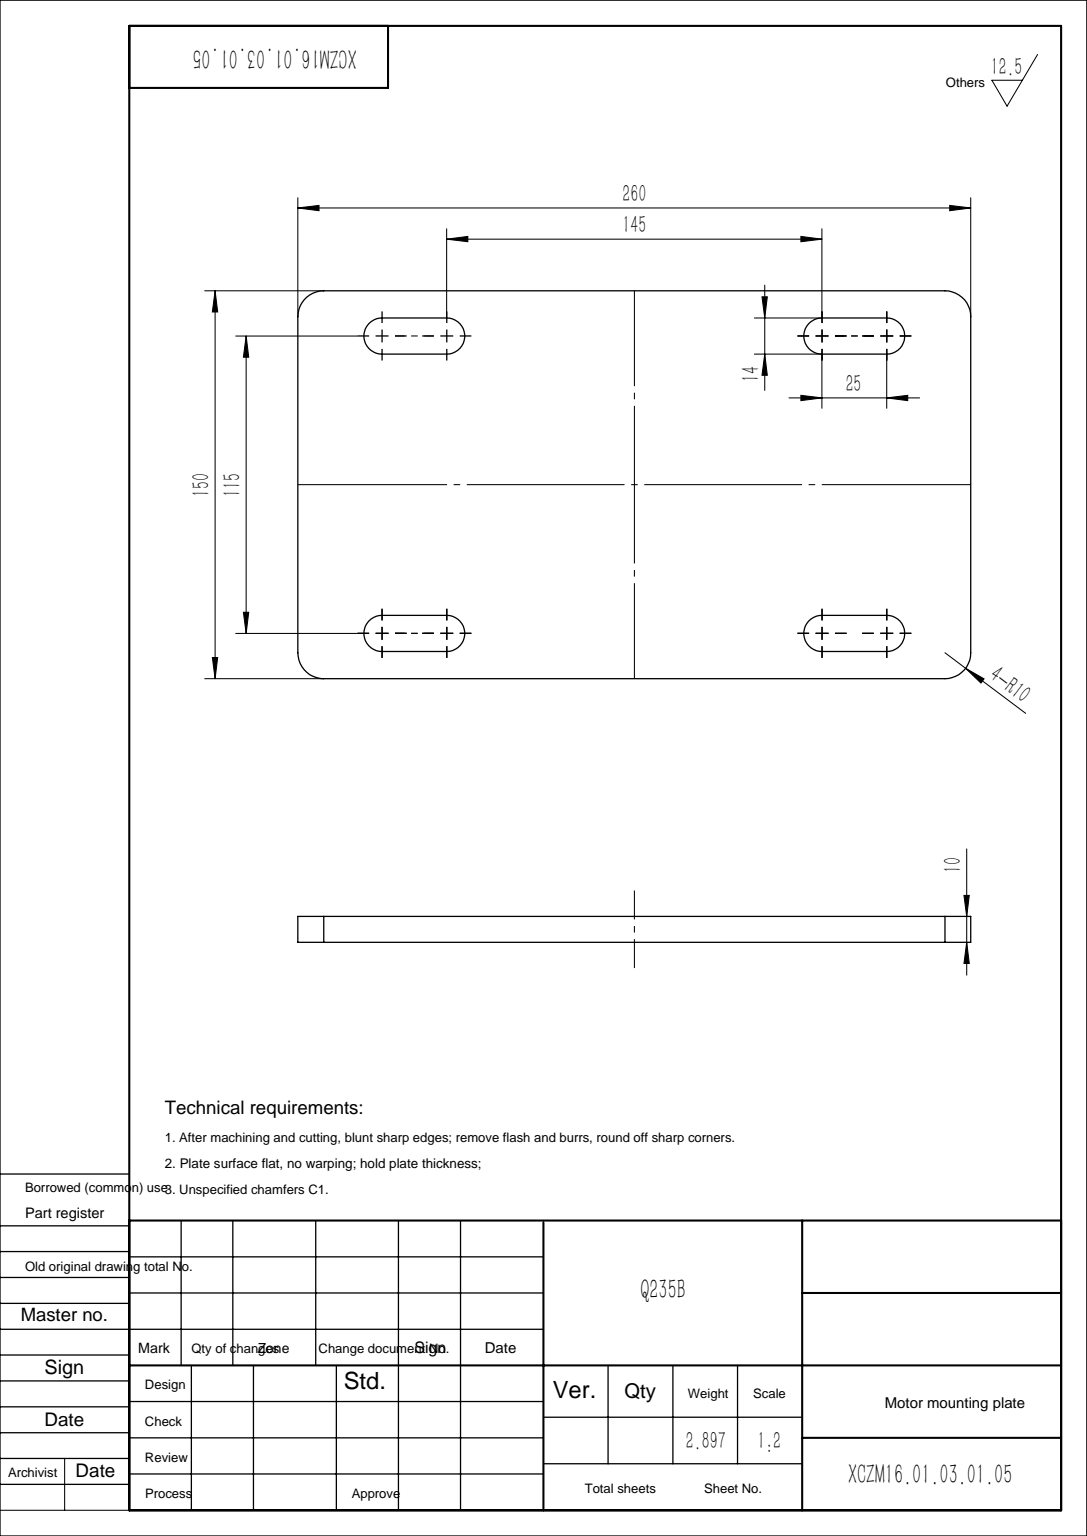
from build123d import *

# Parameters (mm, degrees)
EXTRUDE_1_DEPTH = 10


with BuildPart() as part:
    # 草图1 → 凸台-拉伸1 (new body)
    with BuildSketch(Plane(origin=(0, 0, 0), x_dir=(1, 0, 0), z_dir=(0, 1, 0))):
        with BuildLine():
            Line((120, -75), (-120, -75))
            ThreePointArc((-120, -75), (-127.071067812, -72.071067812), (-130, -65))
            Line((-130, -65), (-130, 65))
            ThreePointArc((-130, 65), (-127.071067812, 72.071067812), (-120, 75))
            Line((-120, 75), (120, 75))
            ThreePointArc((120, 75), (127.071067812, 72.071067812), (130, 65))
            Line((130, 65), (130, -65))
            ThreePointArc((130, -65), (127.071067812, -72.071067812), (120, -75))
        make_face()
        with BuildLine():
            Line((-72.5, 50.5), (-97.5, 50.5))
            ThreePointArc((-97.5, 50.5), (-104.5, 57.5), (-97.5, 64.5))
            Line((-97.5, 64.5), (-72.5, 64.5))
            ThreePointArc((-72.5, 64.5), (-65.5, 57.5), (-72.5, 50.5))
        make_face(mode=Mode.SUBTRACT)
        with BuildLine():
            Line((72.5, 50.5), (97.5, 50.5))
            ThreePointArc((97.5, 50.5), (104.5, 57.5), (97.5, 64.5))
            Line((97.5, 64.5), (72.5, 64.5))
            ThreePointArc((72.5, 64.5), (65.5, 57.5), (72.5, 50.5))
        make_face(mode=Mode.SUBTRACT)
        with BuildLine():
            Line((-72.5, -50.5), (-97.5, -50.5))
            ThreePointArc((-97.5, -50.5), (-104.5, -57.5), (-97.5, -64.5))
            Line((-97.5, -64.5), (-72.5, -64.5))
            ThreePointArc((-72.5, -64.5), (-65.5, -57.5), (-72.5, -50.5))
        make_face(mode=Mode.SUBTRACT)
        with BuildLine():
            Line((72.5, -50.5), (97.5, -50.5))
            ThreePointArc((97.5, -50.5), (104.5, -57.5), (97.5, -64.5))
            Line((97.5, -64.5), (72.5, -64.5))
            ThreePointArc((72.5, -64.5), (65.5, -57.5), (72.5, -50.5))
        make_face(mode=Mode.SUBTRACT)
    extrude(amount=EXTRUDE_1_DEPTH)


solid = part.part
